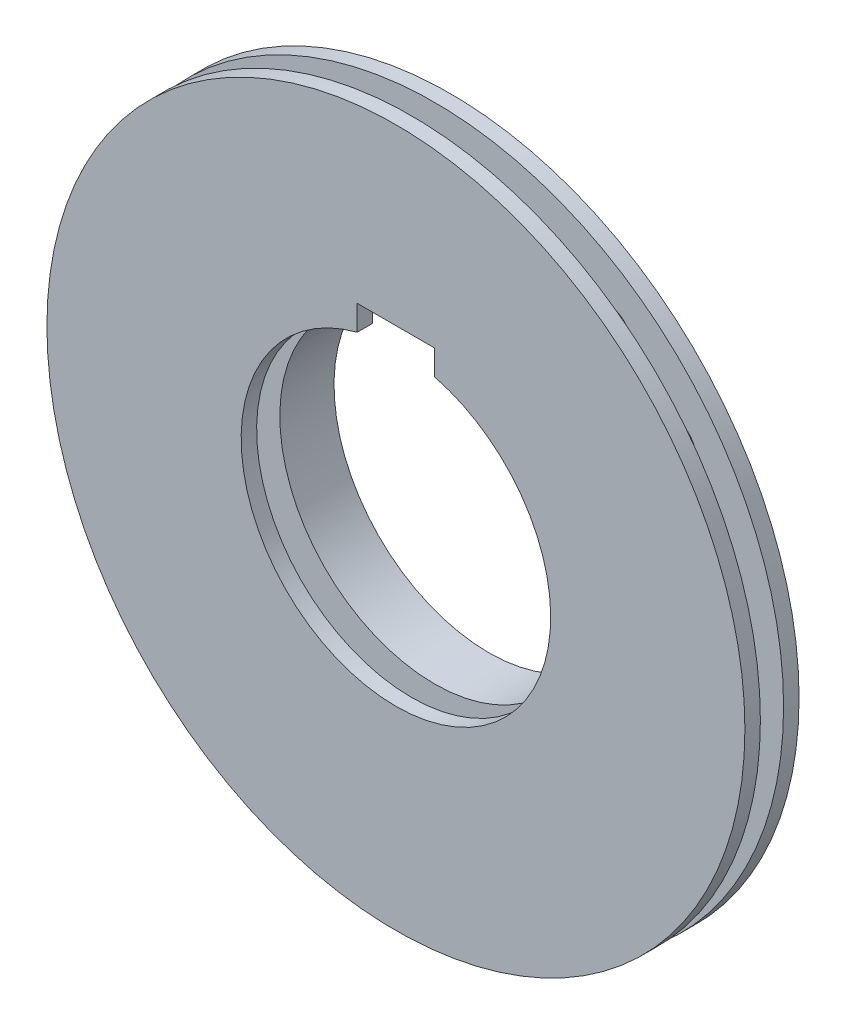
from build123d import *

# Parameters (mm, degrees)
BOSS_EXTRUDE1_START = 7.5
SKETCH1_R           = 225.5
SKETCH1_R_2         = 100
BOSS_EXTRUDE1_DEPTH = 10
SKETCH2_R           = 15
BOSS_EXTRUDE2_DEPTH = 15
SKETCH3_W           = 50
SKETCH3_H           = 48.595629982
CUT_EXTRUDE1_DEPTH  = 321.820043015
SKETCH4_R           = 130
BOSS_EXTRUDE3_DEPTH = 25


with BuildPart() as part:
    # Sketch1 → Boss-Extrude1 (new body)
    with BuildSketch(Plane.XY.offset(BOSS_EXTRUDE1_START)):
        Circle(SKETCH1_R)
        Circle(SKETCH1_R_2, mode=Mode.SUBTRACT)
    extrude(amount=BOSS_EXTRUDE1_DEPTH)


with BuildPart() as body_2:
    # Mirror1: mirrored copy
    add(part.part.mirror(Plane.XY))


with BuildPart() as part_1:
    add(part.part)

    add(body_2.part)  # Boss-Extrude2 merges body 2
    # Sketch2 → Boss-Extrude2 (add)
    with BuildSketch(Plane.XY.offset(-7.5)):
        with Locations((0, 190)):
            Circle(SKETCH2_R)
        with Locations(Location((58.713228931, 180.700738096, 0), (0, 0, 180))):
            Circle(SKETCH2_R)
        with Locations(Location((111.679197936, 153.713228931, 0), (0, 0, 180))):
            Circle(SKETCH2_R)
        with Locations(Location((153.713228931, 111.679197936, 0), (0, 0, 180))):
            Circle(SKETCH2_R)
        with Locations(Location((180.700738096, 58.713228931, 0), (0, 0, 180))):
            Circle(SKETCH2_R)
        with Locations(Location((190, 0, 0), (0, 0, 180))):
            Circle(SKETCH2_R)
        with Locations(Location((180.700738096, -58.713228931, 0), (0, 0, 180))):
            Circle(SKETCH2_R)
        with Locations(Location((153.713228931, -111.679197936, 0), (0, 0, 180))):
            Circle(SKETCH2_R)
        with Locations(Location((111.679197936, -153.713228931, 0), (0, 0, 180))):
            Circle(SKETCH2_R)
        with Locations(Location((58.713228931, -180.700738096, 0), (0, 0, 180))):
            Circle(SKETCH2_R)
        with Locations(Location((0, -190, 0), (0, 0, 180))):
            Circle(SKETCH2_R)
        with Locations(Location((-58.713228931, -180.700738096, 0), (0, 0, 180))):
            Circle(SKETCH2_R)
        with Locations(Location((-111.679197936, -153.713228931, 0), (0, 0, 180))):
            Circle(SKETCH2_R)
        with Locations(Location((-153.713228931, -111.679197936, 0), (0, 0, 180))):
            Circle(SKETCH2_R)
        with Locations(Location((-180.700738096, -58.713228931, 0), (0, 0, 180))):
            Circle(SKETCH2_R)
        with Locations(Location((-190, 0, 0), (0, 0, 180))):
            Circle(SKETCH2_R)
        with Locations(Location((-180.700738096, 58.713228931, 0), (0, 0, 180))):
            Circle(SKETCH2_R)
        with Locations(Location((-153.713228931, 111.679197936, 0), (0, 0, 180))):
            Circle(SKETCH2_R)
        with Locations(Location((-111.679197936, 153.713228931, 0), (0, 0, 180))):
            Circle(SKETCH2_R)
        with Locations(Location((-58.713228931, 180.700738096, 0), (0, 0, 180))):
            Circle(SKETCH2_R)
    extrude(amount=BOSS_EXTRUDE2_DEPTH)

    # Sketch3 → Cut-Extrude1 (cut, through all)
    with BuildSketch(Plane.XY.offset(17.5)):
        with Locations((0, 88.702185009)):
            Rectangle(SKETCH3_W, SKETCH3_H)
    extrude(amount=-CUT_EXTRUDE1_DEPTH, mode=Mode.SUBTRACT)

    # Sketch4 → Boss-Extrude3 (add)
    with BuildSketch(Plane(origin=(0, 0, -17.5), x_dir=(-1, 0, 0), z_dir=(0, 0, -1))):
        Circle(SKETCH4_R)
        with BuildLine():
            Line((-25, 113), (25, 113))
            Line((25, 113), (25, 96.824583655))
            ThreePointArc((25, 96.824583655), (0, -100), (-25, 96.824583655))
            Line((-25, 96.824583655), (-25, 113))
        make_face(mode=Mode.SUBTRACT)
    extrude(amount=BOSS_EXTRUDE3_DEPTH)


solid = part_1.part
